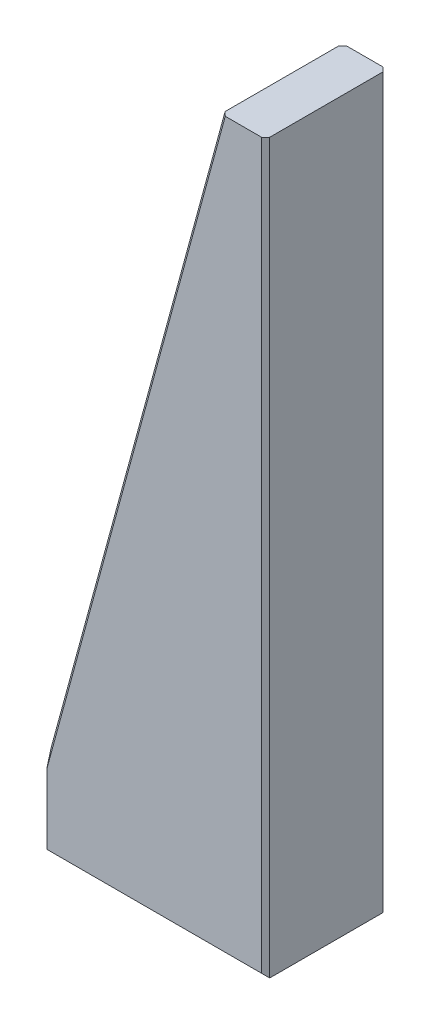
SolidWorks part; units mm, degrees
material "45#"
ref_plane "前视基准面" through (0, 0, 0) normal (0, 0, 1) x (1, 0, 0)
ref_plane "上视基准面" through (0, 0, 0) normal (0, 1, 0) x (1, 0, 0)
ref_plane "右视基准面" through (0, 0, 0) normal (1, 0, 0) x (0, 0, -1)
sketch "草图1" plane through (0, 0, 0) normal (0, 0, 1) x (1, 0, 0)
  line L0 (0, 0) -> (30, 0)
  line L1 (30, 0) -> (30, 110)
  line L2 (30, 110) -> (0, 0)
  dimension "D1" = 30
  dimension "D2" = 110
extrude "凸台-拉伸1" add sketch "草图1" along normal blind 15
chamfer "倒角1" distance 0.5 angle 45 6 edges at (30, 55, 0) (15, 55, 0) (15, 0, 0) (30, 55, 15) (15, 0, 15) (15, 55, 15)
sketch "草图7" plane through (0, 0, 15) normal (0, 0, 1) x (1, 0, 0)
  line L0 (0, 0) -> (30, 110) construction
  line L1 (30, 110) -> (24.5, 110)
  line L2 (30, 110) -> (30, 89.8333)
  line L3 (30, 89.8333) -> (24.5, 89.8333)
  line L4 (24.5, 110) -> (24.5, 89.8333)
  line L5 (0, 0) -> (3, 0)
  line L6 (0, 0) -> (0, 20)
  line L7 (0, 20) -> (3, 20)
  line L8 (3, 0) -> (3, 20)
  dimension "D1" = 5.5
  dimension "D3" = 3
  dimension "D4" = 20
extrude "切除-拉伸1" cut sketch "草图7" against normal through all
